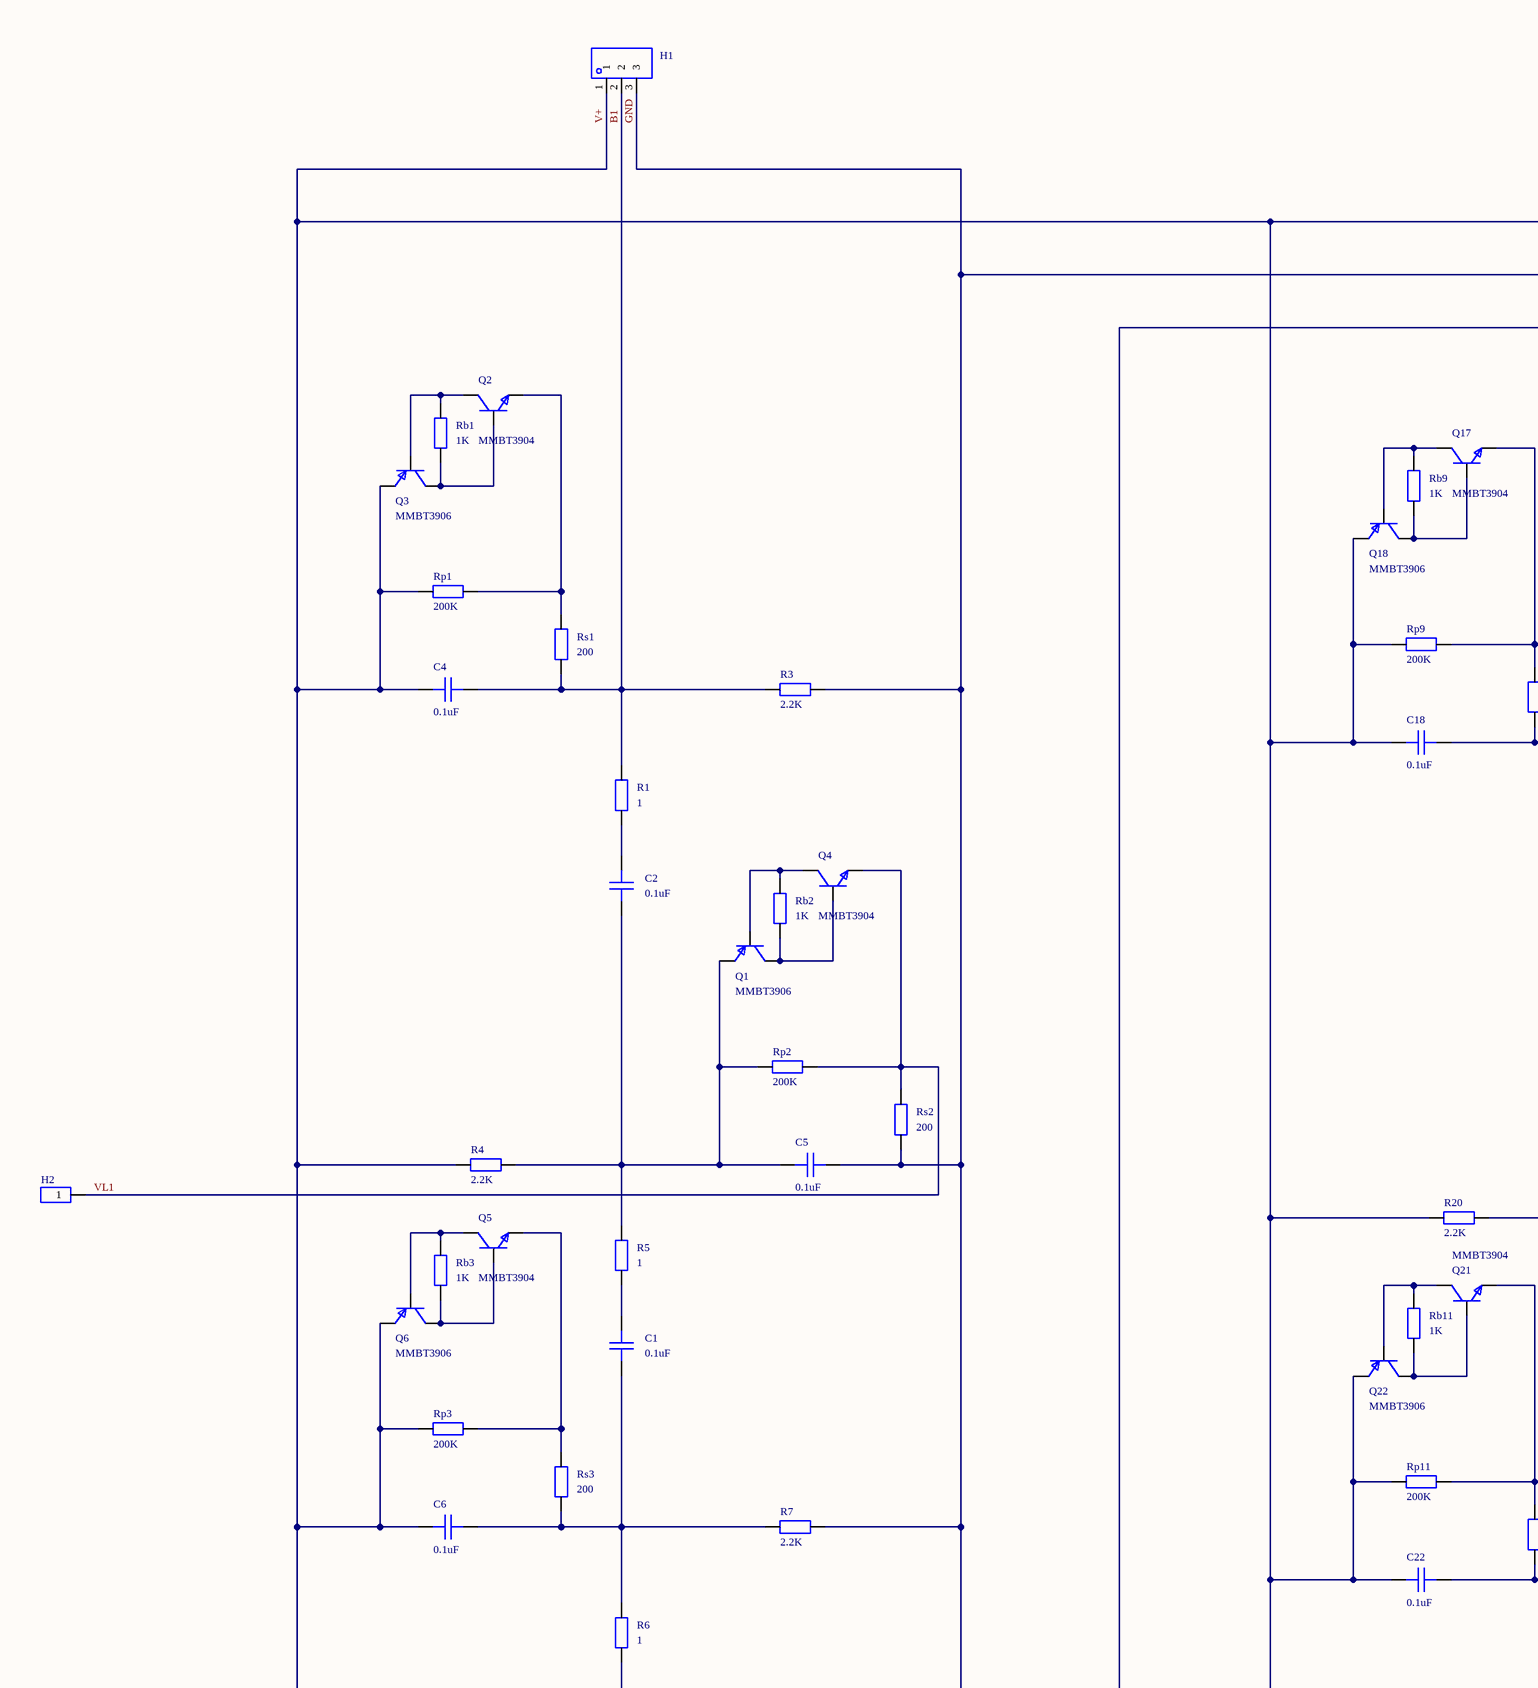
[diagram p0: MISC61260-3.schdoc, top left]
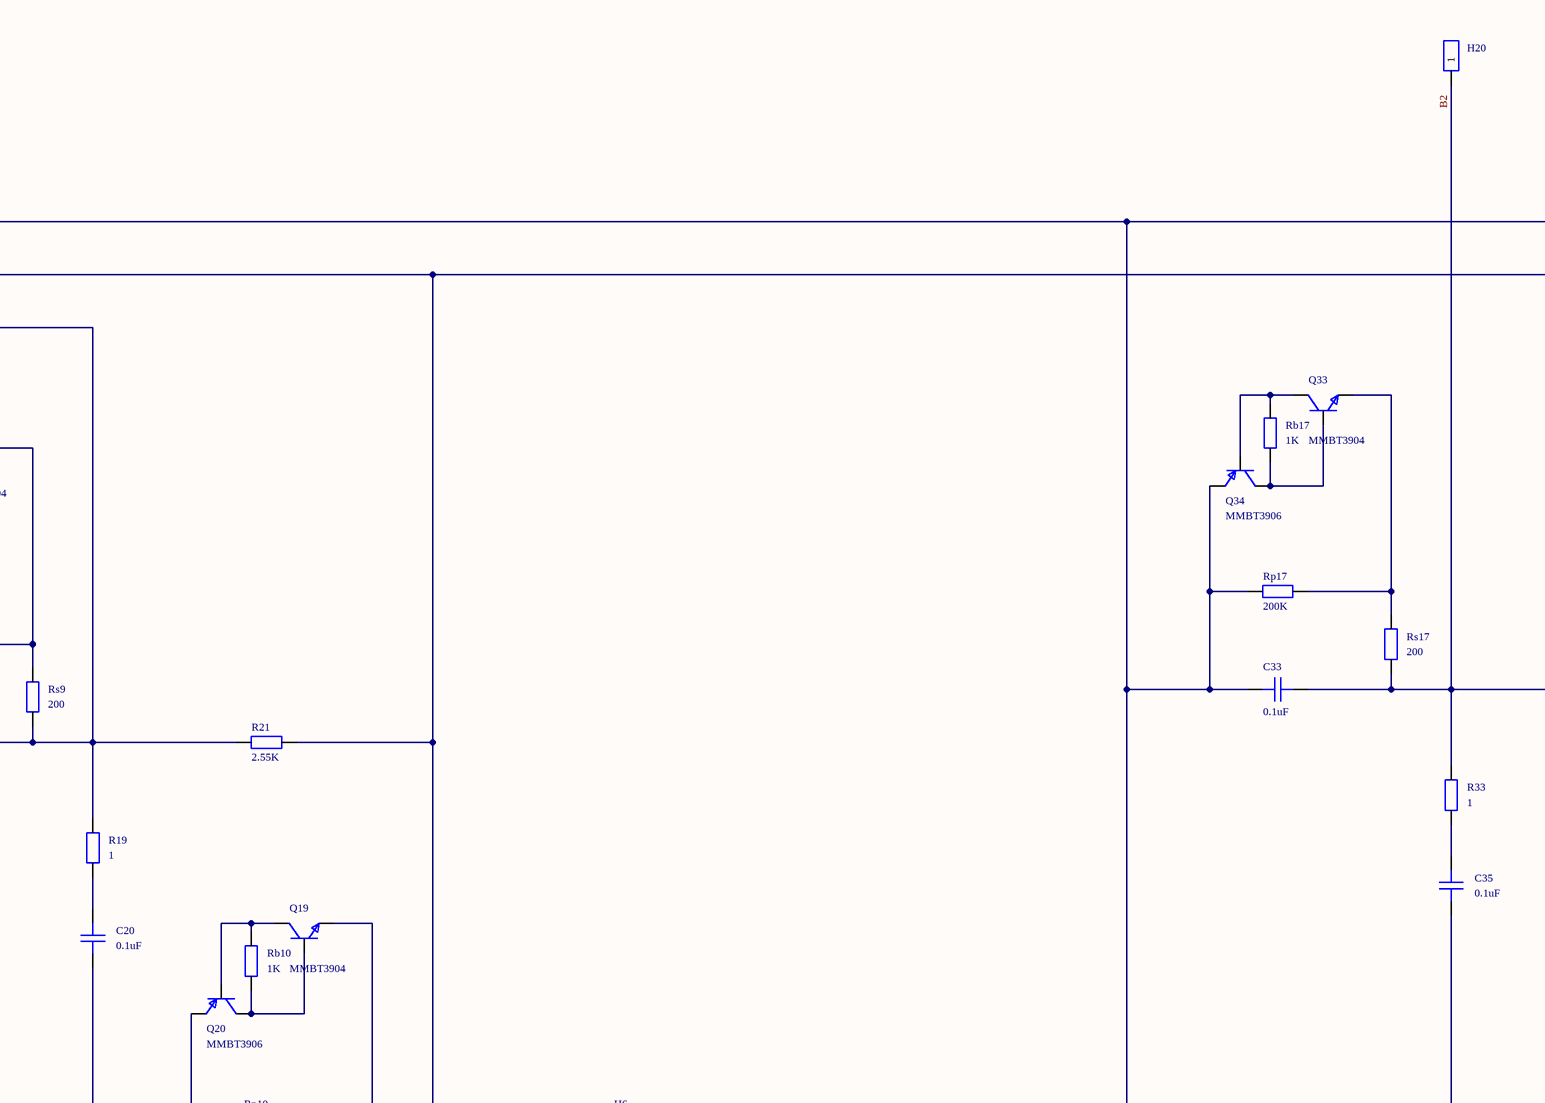
[diagram p1: MISC61260-3.schdoc, top middle]
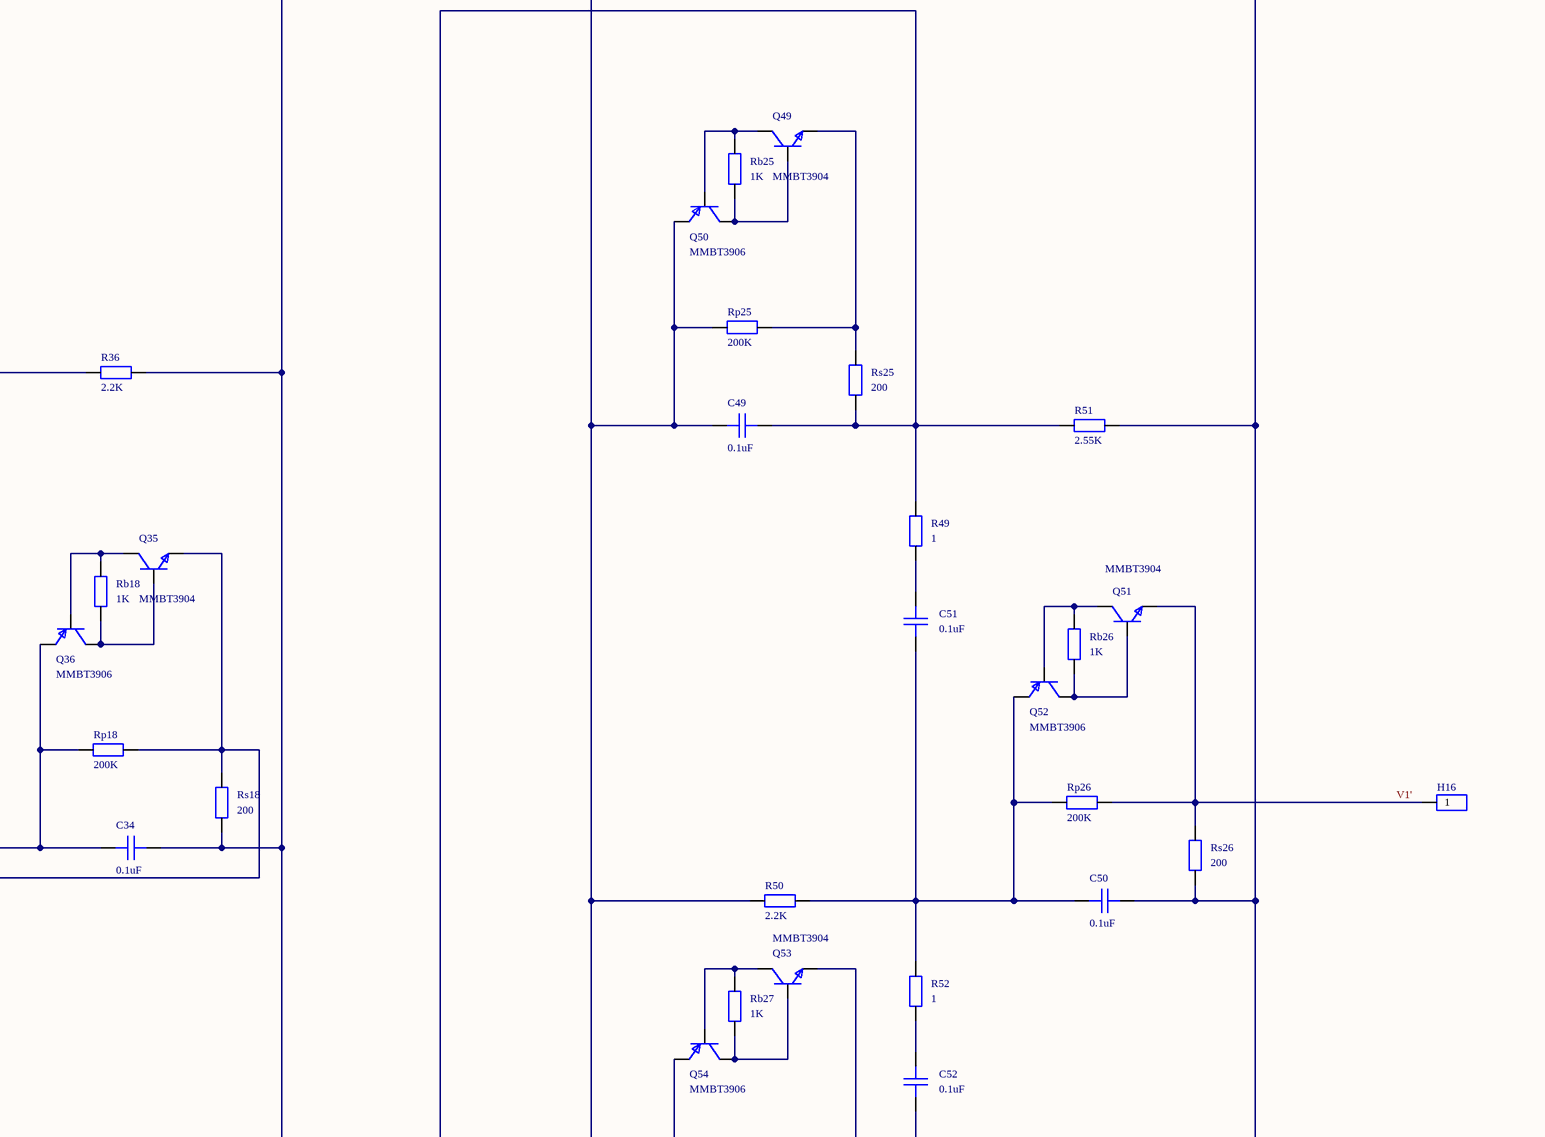
[diagram p2: MISC61260-3.schdoc, top right]
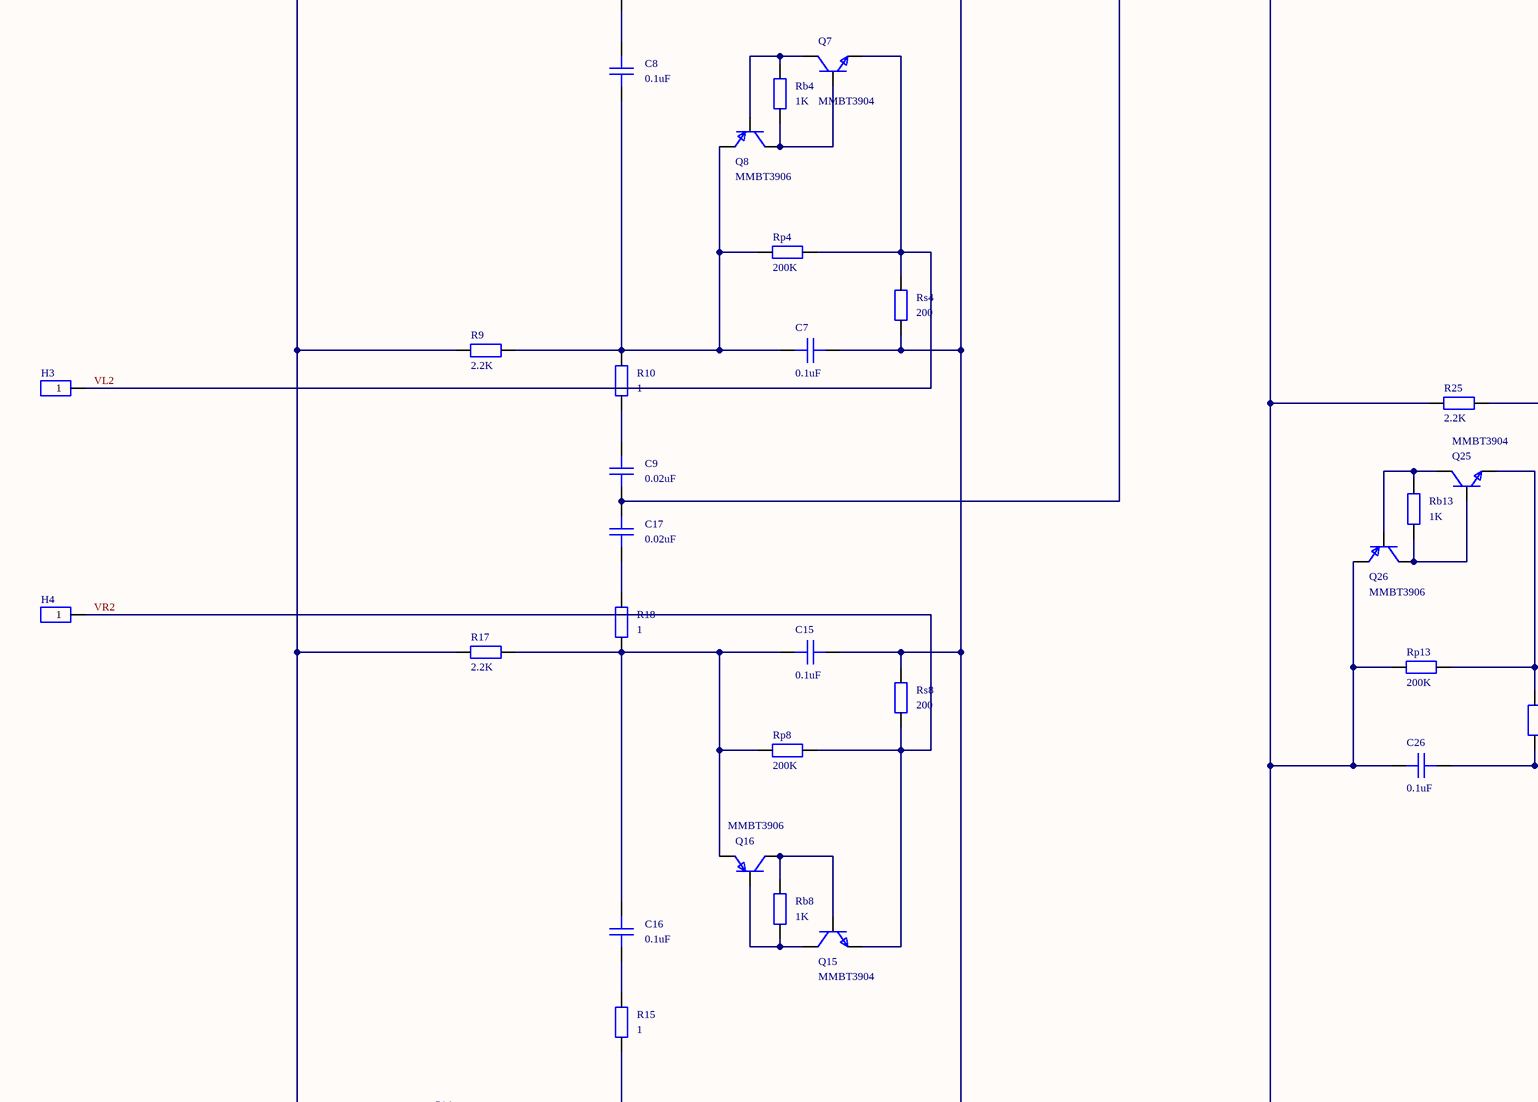
[diagram p3: MISC61260-3.schdoc, centre left]
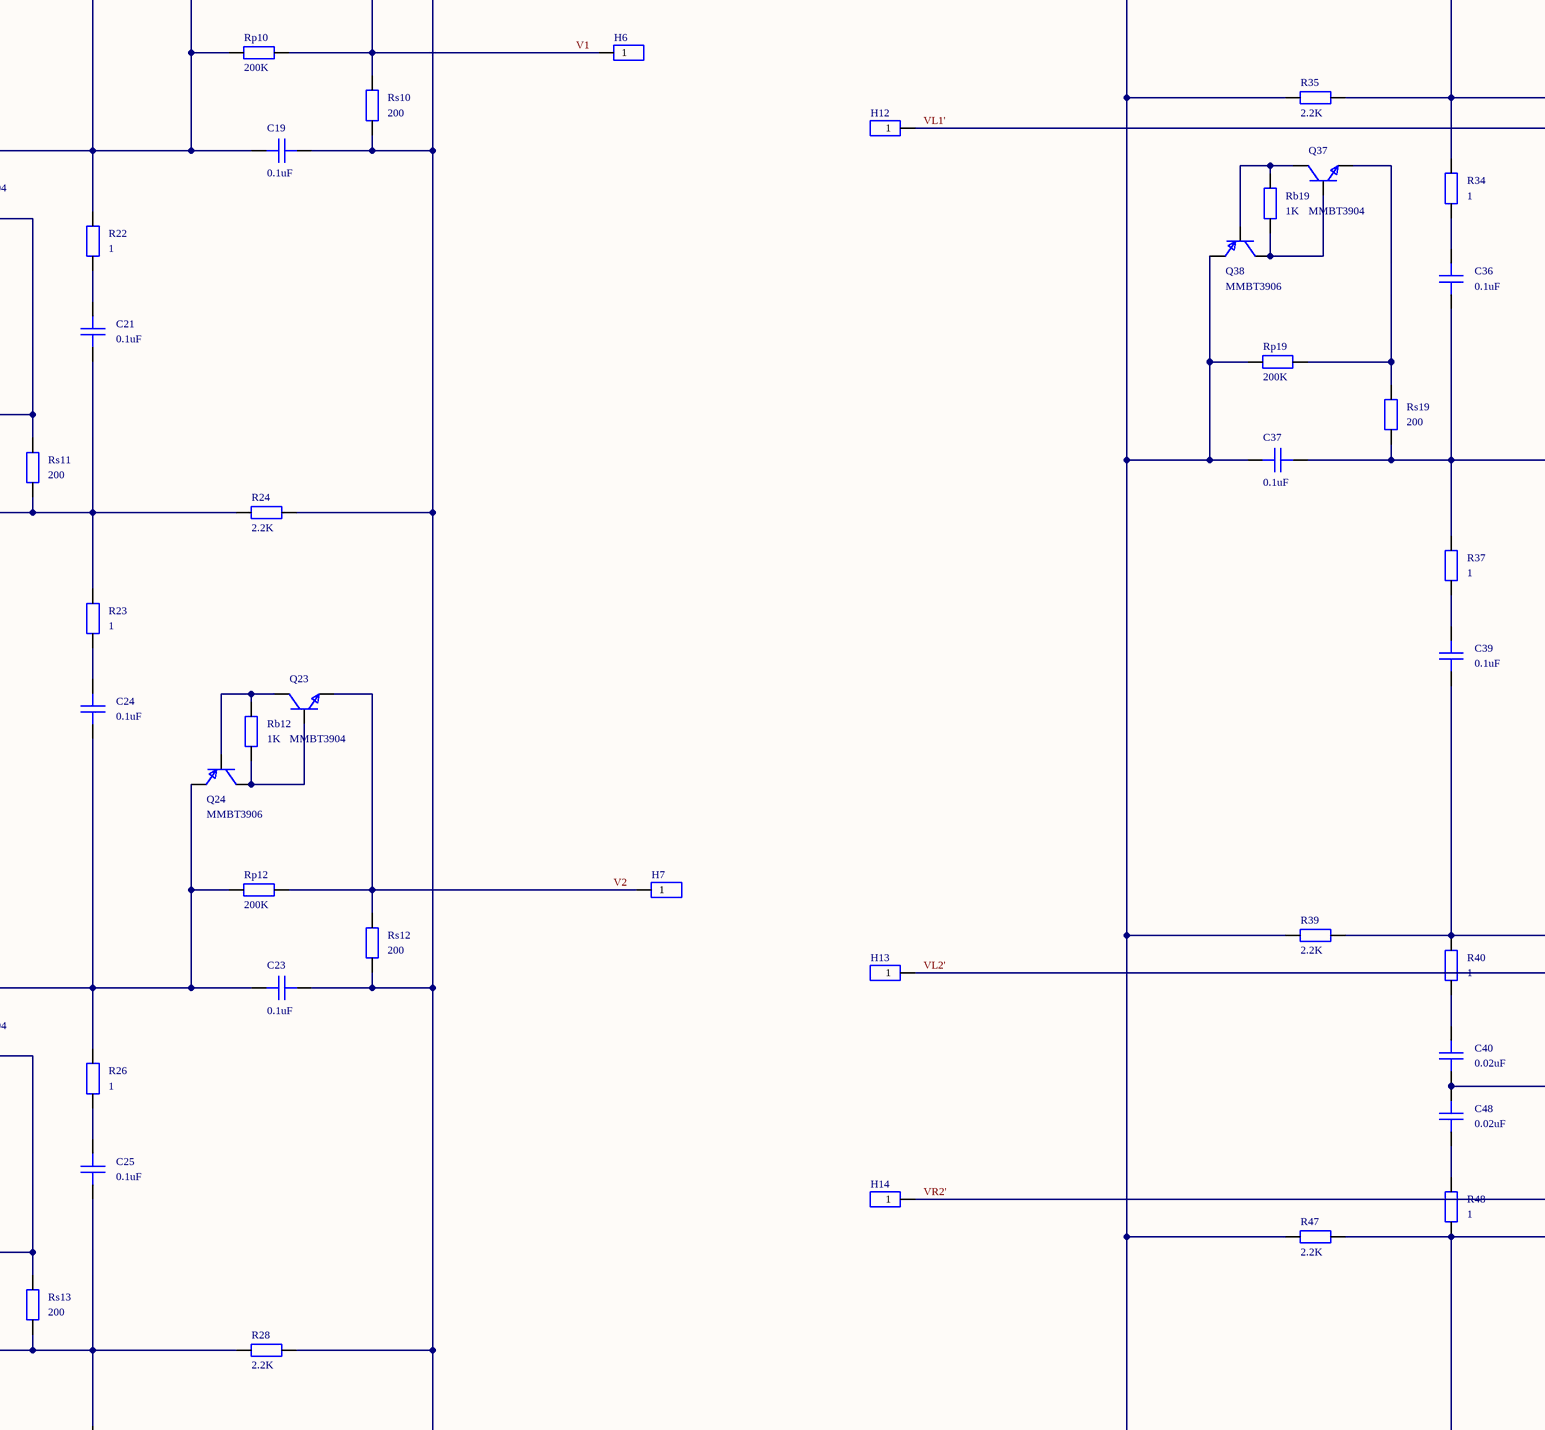
[diagram p4: MISC61260-3.schdoc, centre middle]
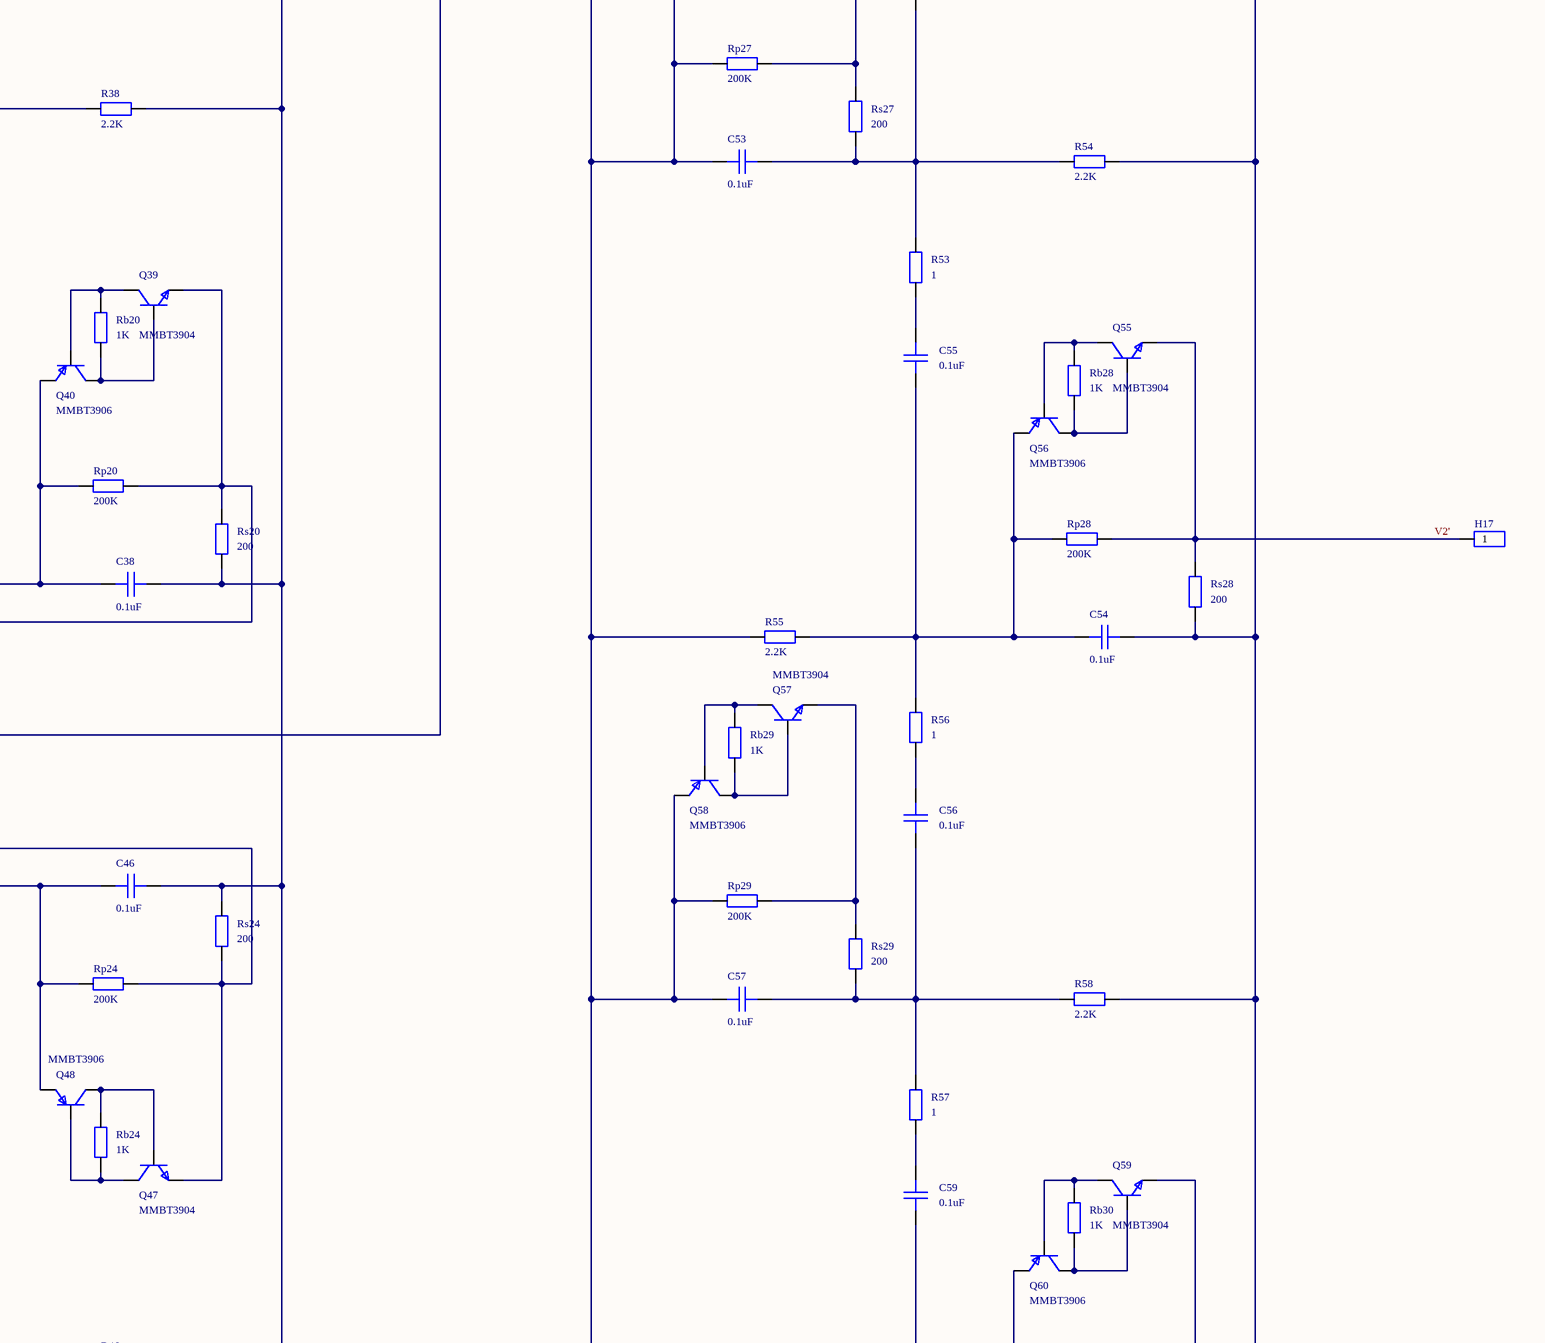
[diagram p5: MISC61260-3.schdoc, centre right]
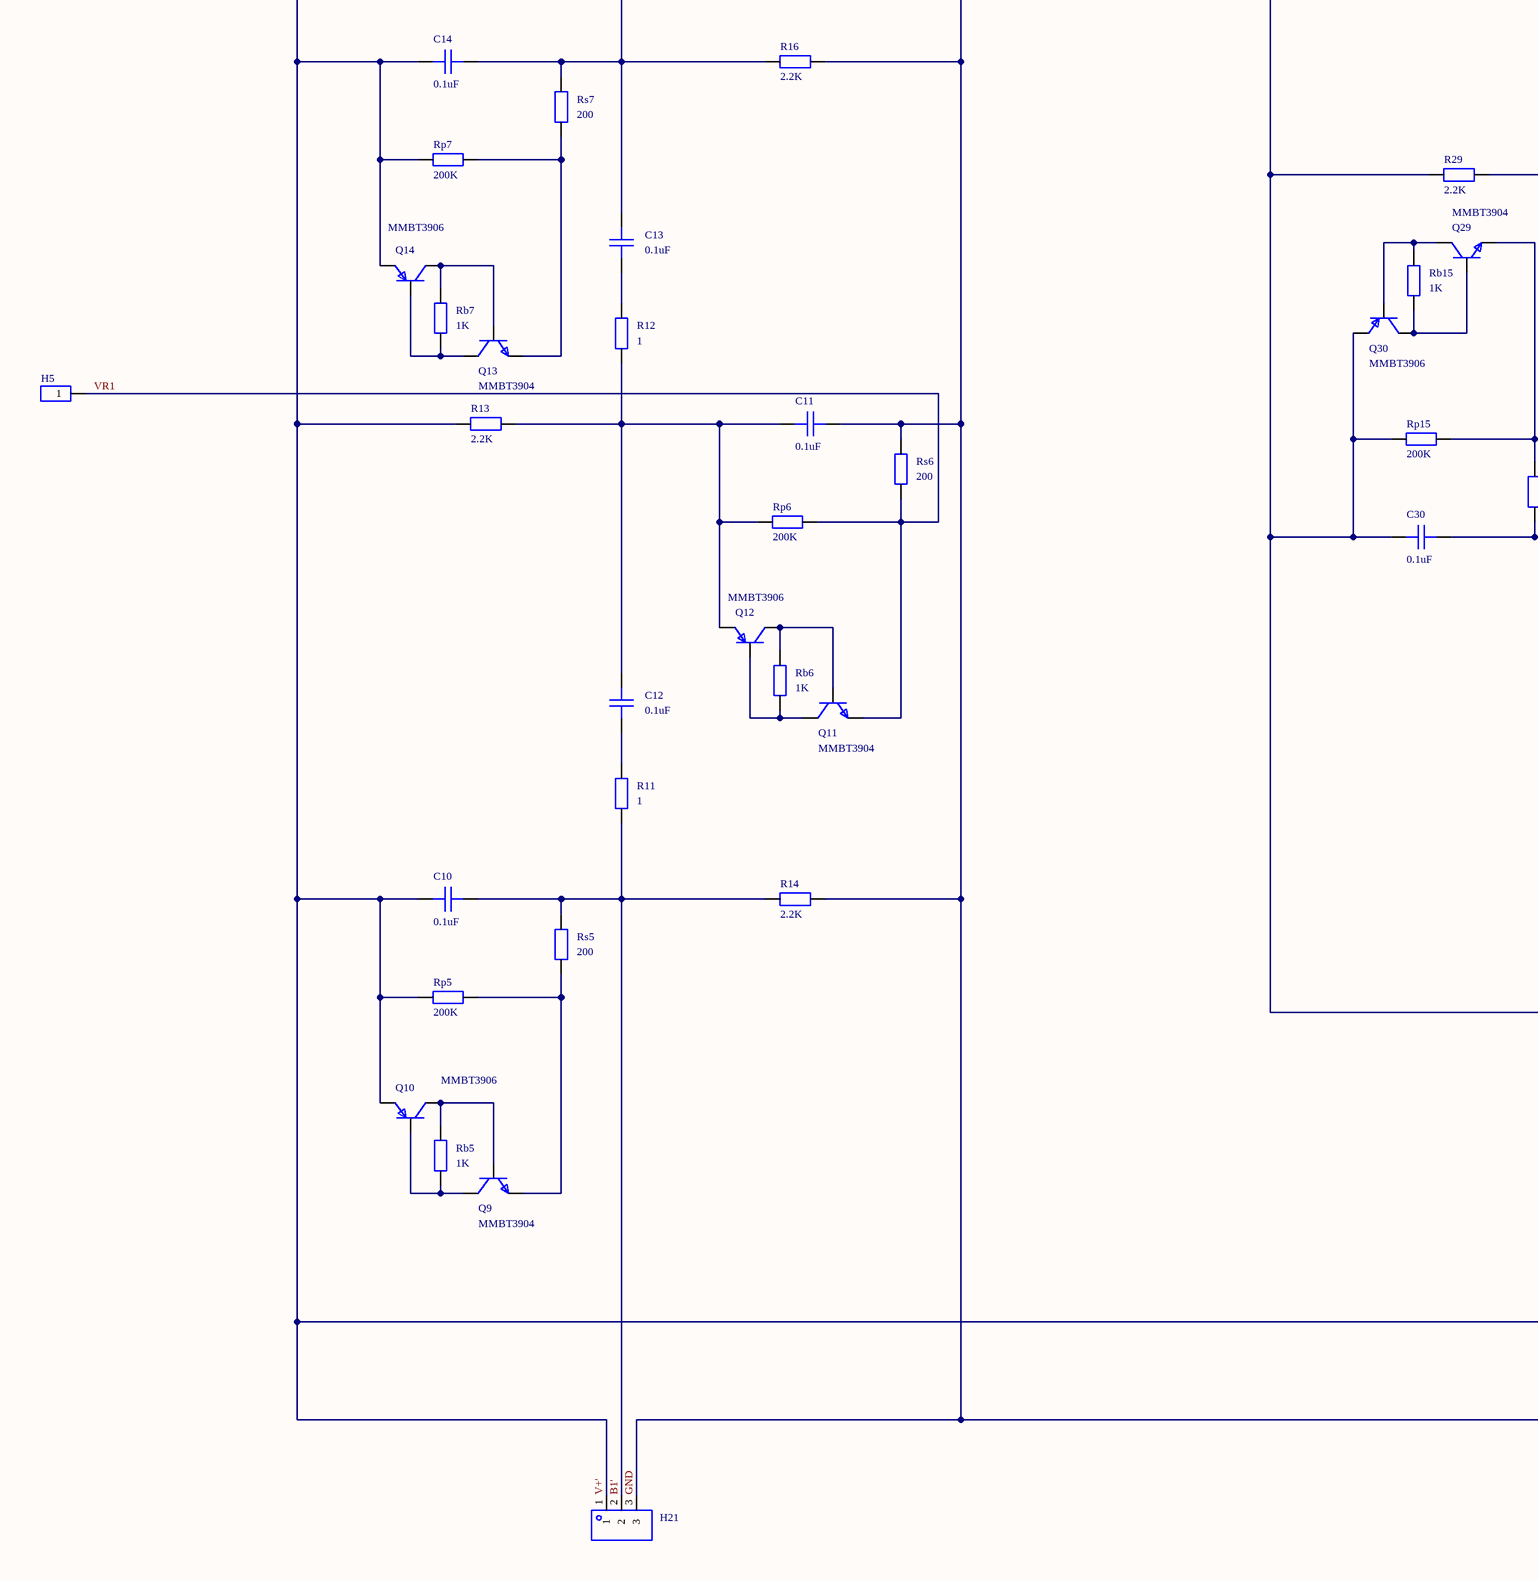
[diagram p6: MISC61260-3.schdoc, bottom left]
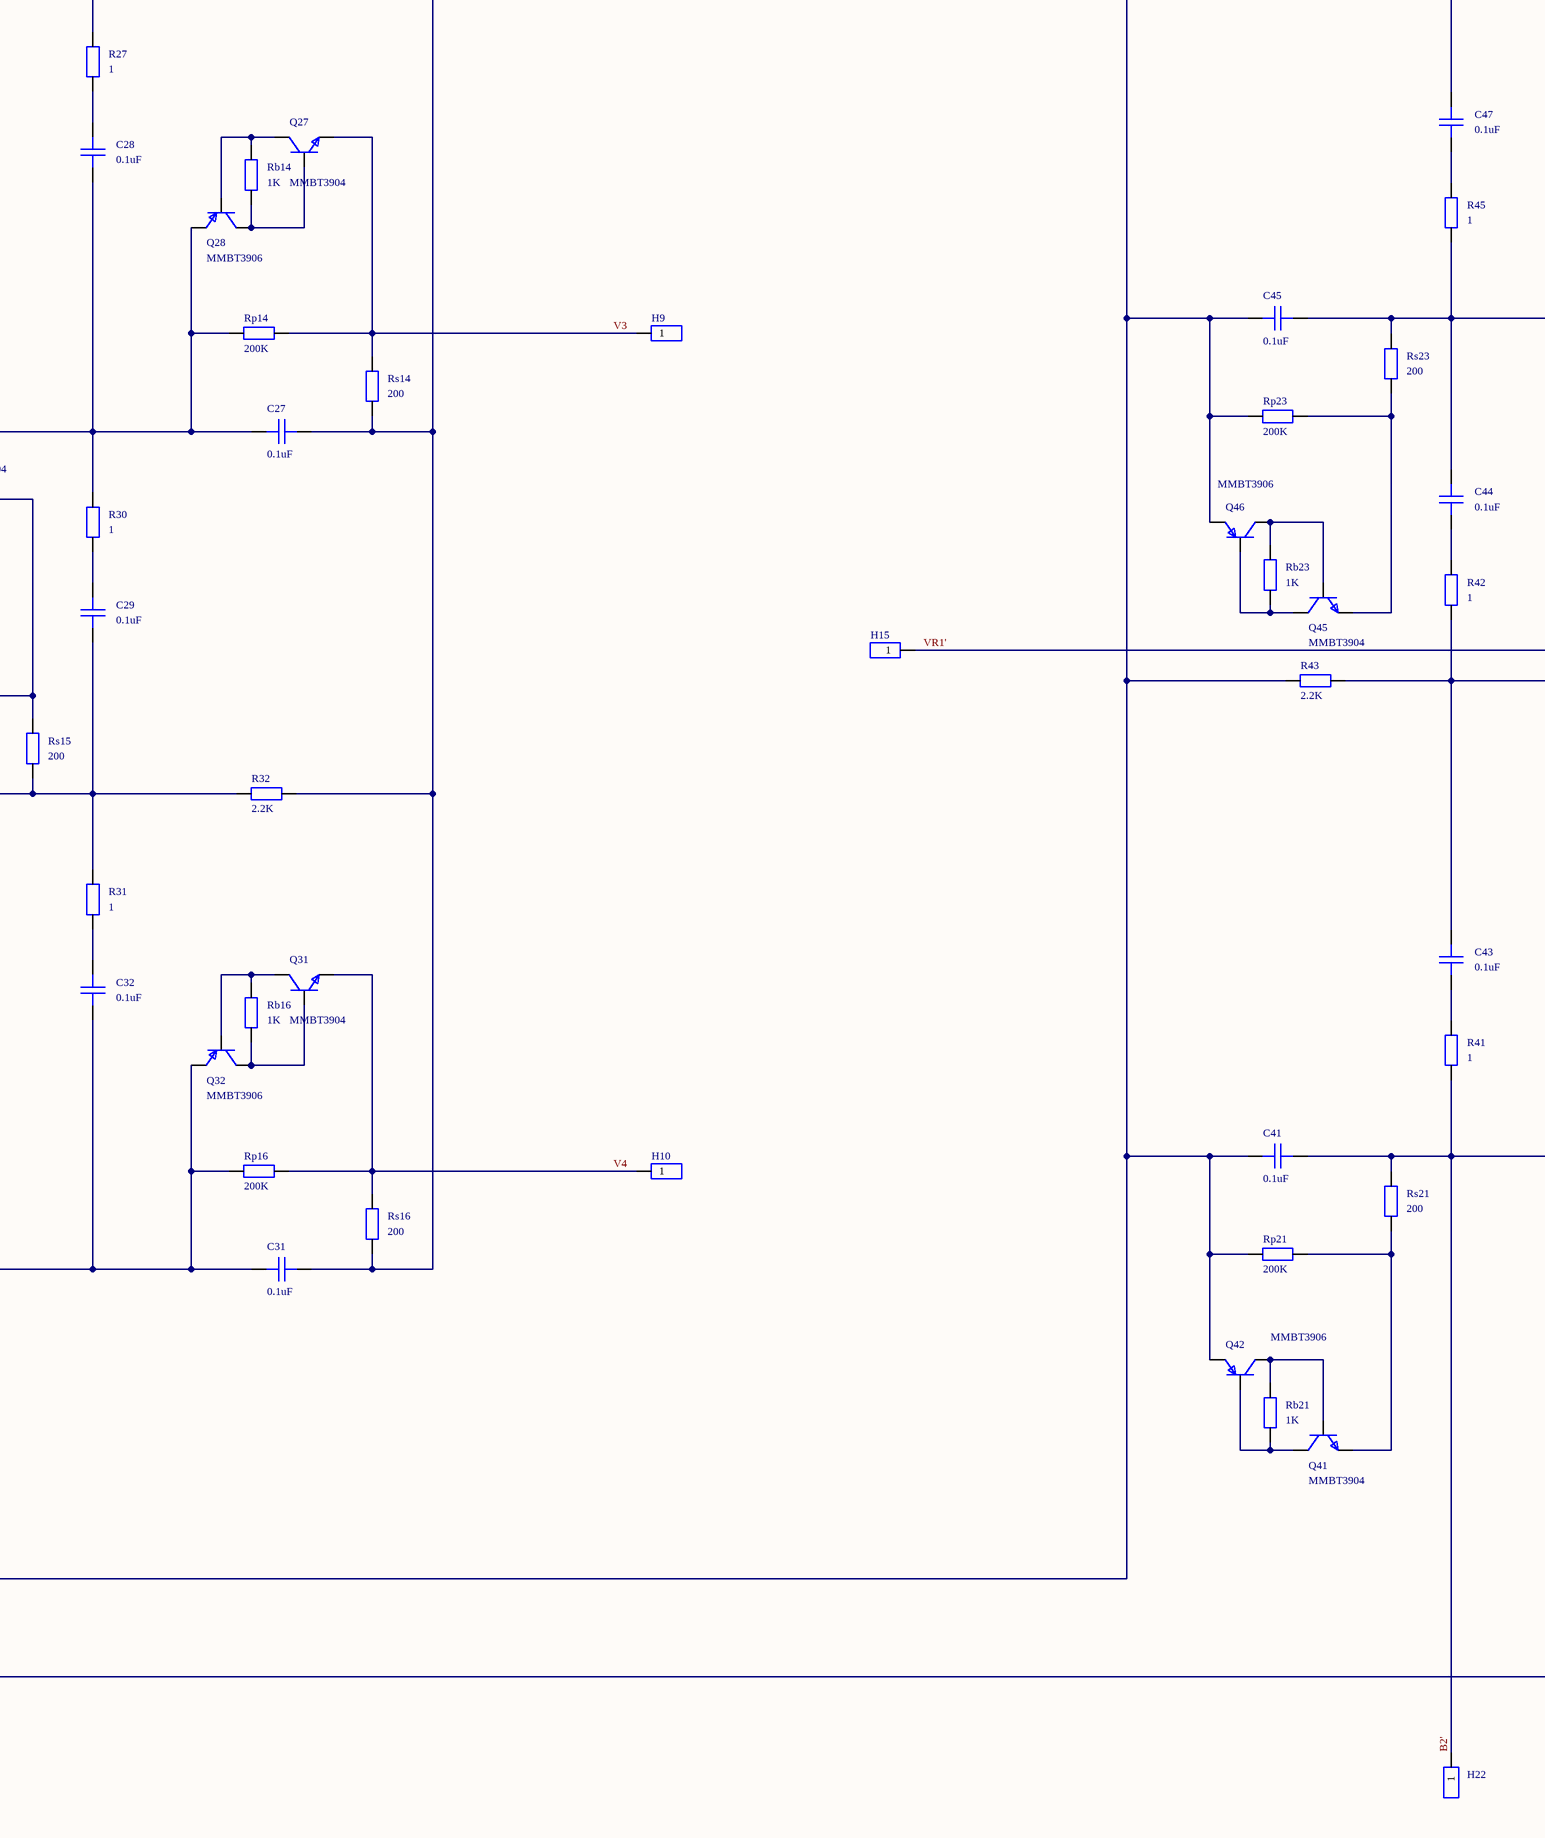
[diagram p7: MISC61260-3.schdoc, bottom middle]
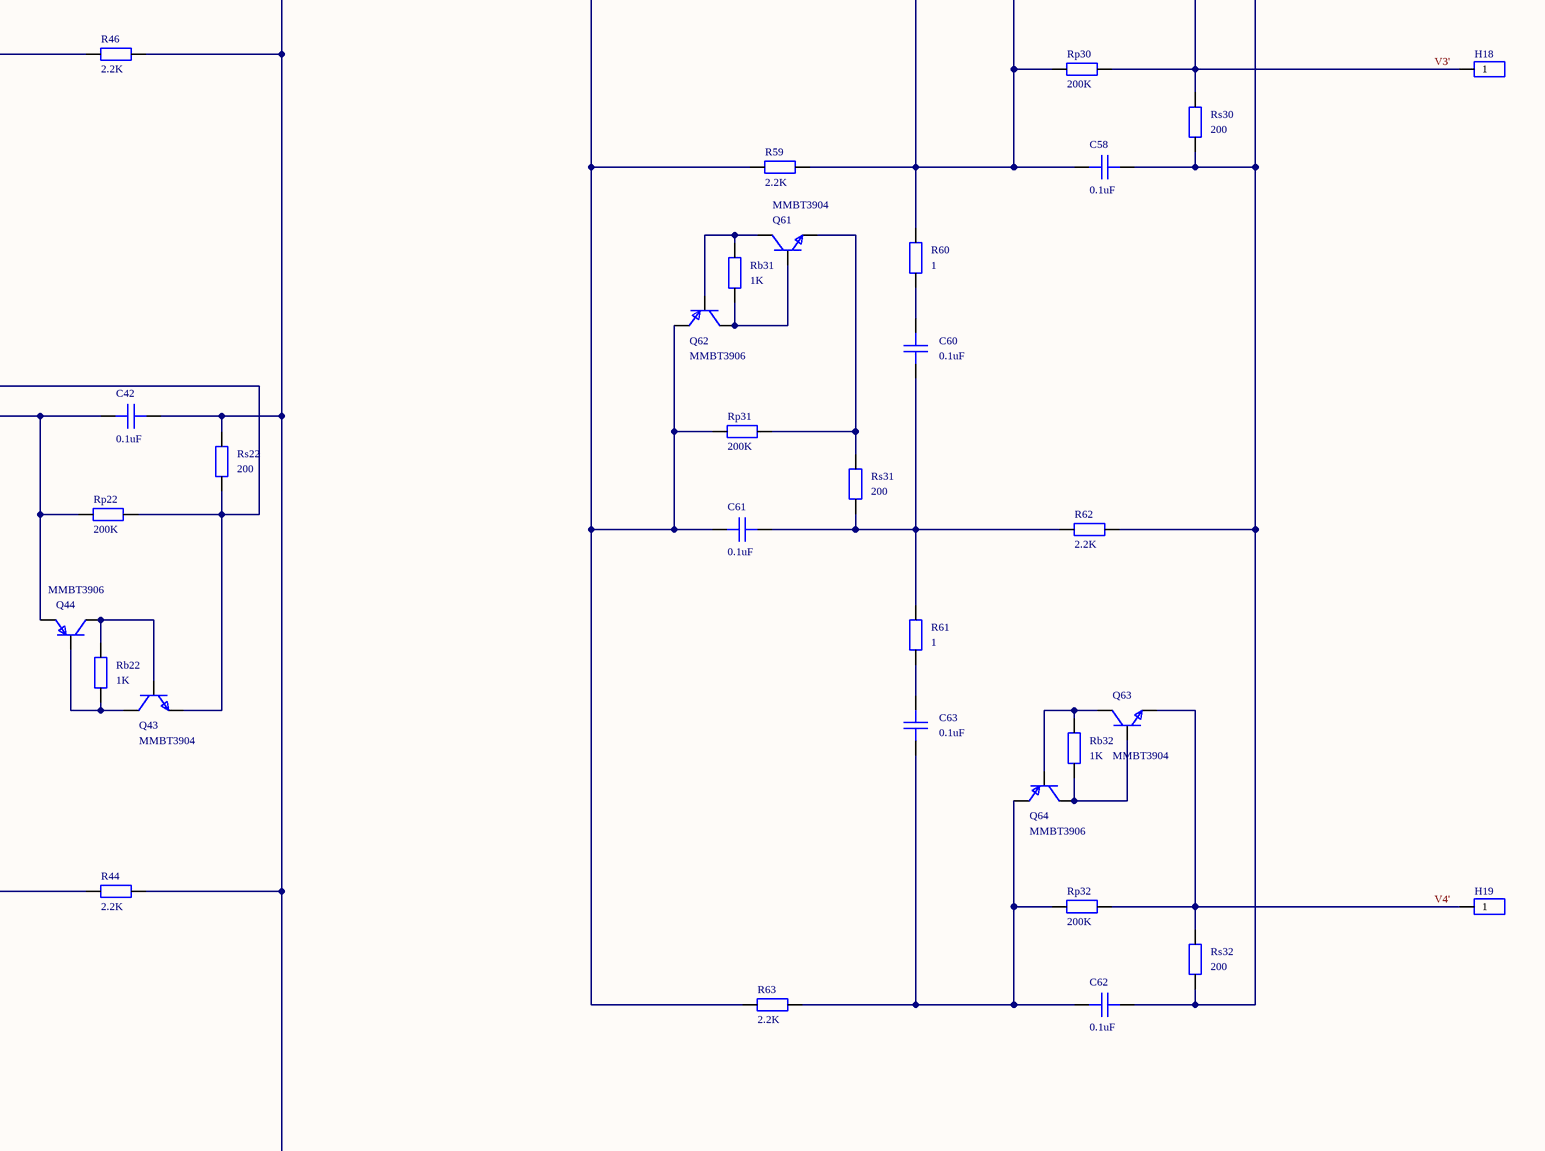
[diagram p8: MISC61260-3.schdoc, bottom right]
# Altium project MISC61260-2.PrjPcb (part 1 of 2)
1 sheet, 303 parts. Net scope: global (net labels, ports and power ports of the same name join across sheets).
Board file: MISC61260.pcbdoc